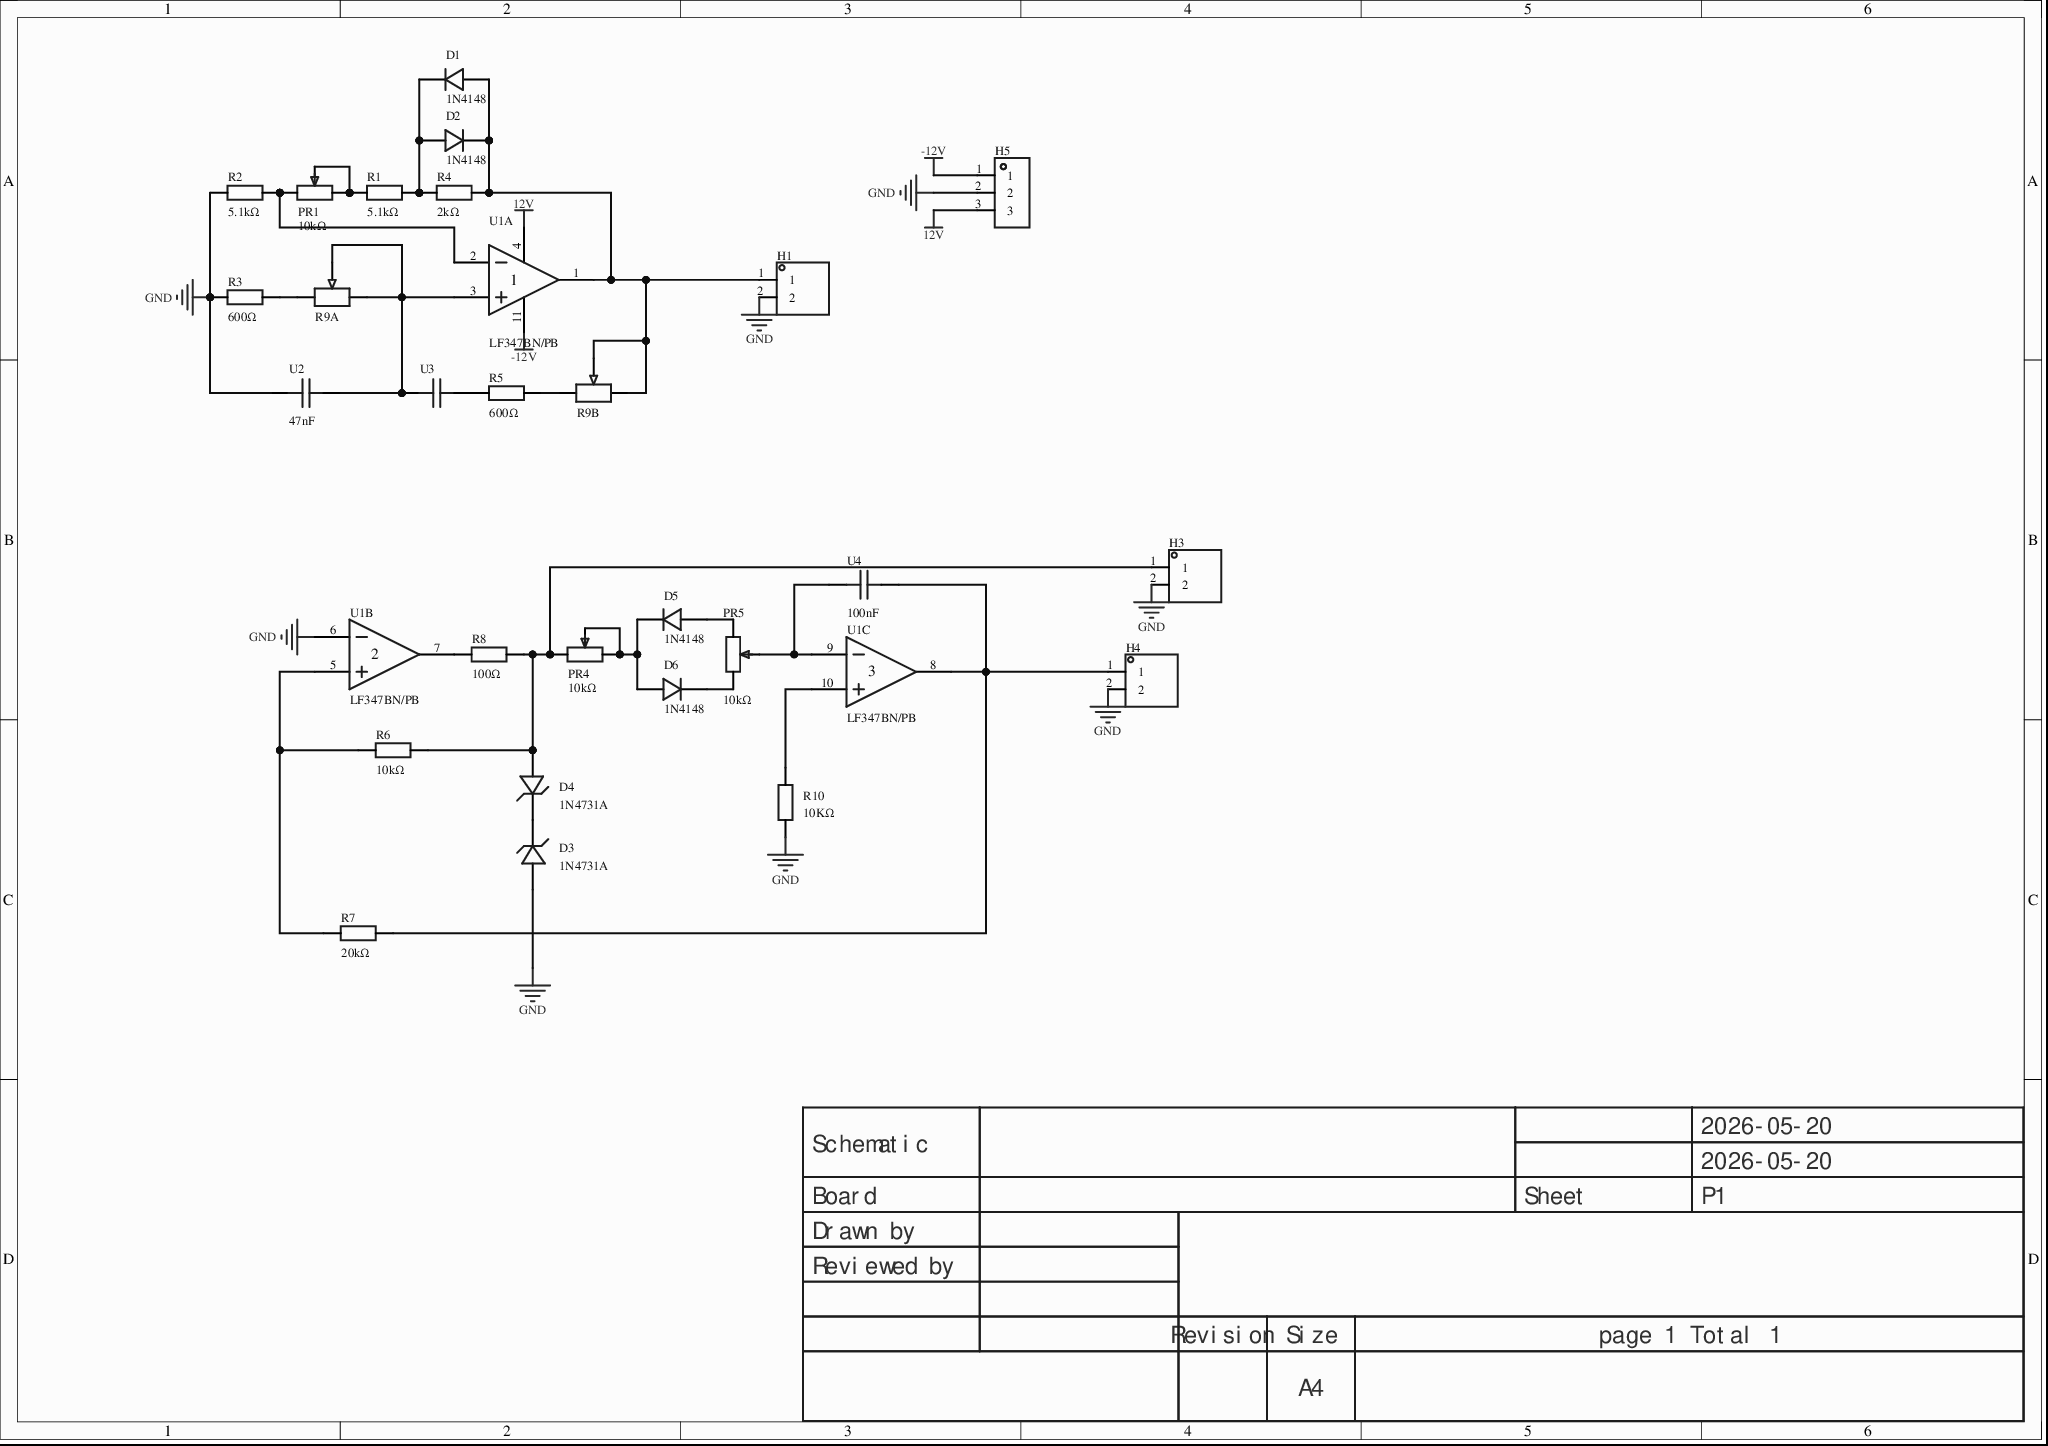
[diagram p0: MISC89085-3.schdoc]
# Altium project MISC89085-2.PrjPcb
1 sheet, 27 parts. Net scope: global (net labels, ports and power ports of the same name join across sheets).
Board file: MISC89085.pcbdoc

## Sheet MISC89085-3.schdoc
size 297 x 209 mm; Version: V1.0; @Project Name: MISC89085; @Update Date: 2026-05-20; @Create Date: 2026-05-20; @Board Name: MISC89085; @Create Time: 18:00:22; @Page Count: 1; @Page No: 1; @Schematic Name: MISC89085; @Update Time: 18:00:22; Size: A4

### Parts
D1  1N4148  [DO-35_BD2.2-L4.0-D0.50_1N4148]
D2  1N4148  [DO-35_BD2.2-L4.0-D0.50_1N4148]
D3  1N4731A  [DO-41_BD2.4-L4.7-P8.70-D0.9-RD]
D4  1N4731A  [DO-41_BD2.4-L4.7-P8.70-D0.9-RD]
D5  1N4148  [DO-35_BD2.2-L4.0-D0.50_1N4148]
D6  1N4148  [DO-35_BD2.2-L4.0-D0.50_1N4148]
H1  (no value)  [HDR-TH_2P-P2.54-V-M-1]
H3  (no value)  [HDR-TH_2P-P2.54-V-M-1]
H4  (no value)  [HDR-TH_2P-P2.54-V-M-1]
H5  (no value)  [HDR-TH_3P-P2.54-V-M]
PR1  10kΩ  [R_3296]
PR4  10kΩ  [R_3296]
PR5  10kΩ  [R_3296]
R1  5.1kΩ  [Res_1/8W]
R2  5.1kΩ  [Res_1/8W]
R3  600Ω  [Res_1/8W]
R4  2kΩ  [Res_1/8W]
R5  600Ω  [Res_1/8W]
R6  10kΩ  [Res_1/8W]
R7  20kΩ  [Res_1/8W]
R8  100Ω  [Res_1/8W]
R9  (no value)  [WH148]  (parts A,B of 2)
R10  10KΩ  [Res_1/8W]
U1  LF347BN/PB  [PDIP-14_L19.6-W6.5-P2.54-LS7.9-BL]  (parts A,B,C of 4)
U2  47nF  [CAP-TH_L5.0-W2.5-P5.00-D1.0]
U3  47nF  [CAP-TH_L5.0-W2.5-P5.00-D1.0]  (value not drawn)
U4  100nF  [CAP-TH_L5.0-W2.5-P5.00-D1.0]

### Nets
12V: H5.3 U1.4(VCC+)
-12V: H5.1 U1.11(VCC-)
GND: D3.2(A) H1.2 H3.2 H4.2 H5.2 R2.1 R3.1 R10.1 U1.6(IN2-) U2.2
NetD1_1: D1.1(A) D2.2(C) H1.1 R4.2 R9.5 R9.6 U1.1(OUT1)
NetD1_2: D1.2(C) D2.1(A) R1.2 R4.1
NetD3_1: D3.1(C) D4.1(C)
NetD4_2: D4.2(A) H3.1 PR4.3 R6.2 R8.2
NetD5_1: D5.1(A) PR5.3
NetD5_2: D5.2(C) D6.1(A) PR4.1 PR4.2
NetD6_2: D6.2(C) PR5.1
NetH4_1: H4.1 R7.2 U1.8(OUT3) U4.1
NetPR1_1: PR1.1 PR1.2 R1.1
NetPR1_3: PR1.3 R2.2 U1.2(IN1-)
NetPR5_2: PR5.2 U1.9(IN3-) U4.2
NetR3_2: R3.2 R9.3
NetR5_1: R5.1 U3.1
NetR5_2: R5.2 R9.4
NetR6_1: R6.1 R7.1 U1.5(IN2+)
NetR8_1: R8.1 U1.7(OUT2)
NetR9_1: R9.1 R9.2 U1.3(IN1+) U2.1 U3.2
NetR10_2: R10.2 U1.10(IN3+)

### Notes on the sheet
- 2026-05-20
- Schematic
- Board
- Sheet
- P1
- Drawn by
- Reviewed by
- Revision
- Size
- A4
- page 1 Total 1

### Library data of the parts
D1 D2 D5 D6 = 1N4148_C9900036548: AddInBom: yes; ModelId: b29439ed7b924f62acded4384188502f0819f05c4eef4c71ace90d822a990e87; ModelTransform: 334.645,87.008,0,0,0,0,0,0,-196.85; Symbol: 1N4148_C9900036548; Device: 1N4148_C9900036548; LCSC Part Name: 1N4148; SupplierPart: C9900036548; ManufacturerPart: 1N4148; Supplier Footprint: LL34; JLCPCB Part Class: Extended Part; Supplier: LCSC; ConvertToPcb: yes; FootprintName: DO-35_BD2.2-L4.0-D0.50_1N4148; ModelName: DO-35_BD2.2-L4.0-D0.50_1N4148
D3 D4 = 1N4731A: Diode configuration: standalone; Zener voltage (nominal): 4.3V; Zener voltage (range): 4.085V~4.515V; Power (Pd): 1W;; Manufacturer: TC(德昌); Symbol: 1N4731A_C261313; AddInBom: yes; ModelId: 6de1e9b71a0d4751b4e9df530304c1a30819f05c4eef4c71ace90d822a990e87; ModelName: DO-41_D2.4-L4.7-P8.70; ModelTransform: 374.016,94.488,0,0,0,0,0,0,-137.795; Reverse Leakage Current (Ir): 10uA@1V; Zener Impedance (Zzt): 9Ω; Device: 1N4731A; LCSC Part Name: 1N4731A; SupplierPart: C261313; ManufacturerPart: 1N4731A; Supplier Footprint: DO-41; JLCPCB Part Class: Extended Part; Datasheet: example.com/20180730/C261314_DA1057BB6837687397320D9A8FF0874A.pdf; Supplier: LCSC; ConvertToPcb: yes; FootprintName: DO-41_BD2.4-L4.7-P8.70-D0.9-RD; Diode Configuration: Standalone; Zener Voltage (Nom): 4.3V; Zener Voltage (Range): 4.085V~4.515V; Power Dissipation: 1W
H1 H3 H4 = HDR-M_2.54_1x2P: Symbol: 210S-1*2P L=11.6MMGold-plated black; ConvertToPcb: yes; ModelId: 79b2e9f2d70a4d68a1b7098f27c6d4c50819f05c4eef4c71ace90d822a990e87; ModelName: HDR-M-2.54_1x2; ModelTransform: 200,100,0,0,0,0,0,0,-118.11; Device: HDR-M_2.54_1x2P; AddInBom: yes; SupplierPart: C124375; Supplier Footprint: 插件; FootprintName: HDR-TH_2P-P2.54-V-M-1
H5 = HDR-M_2.54_1x3P: AddInBom: yes; ModelId: bb473b6d38ff42a99216a4fcdbdcc4cb0819f05c4eef4c71ace90d822a990e87; ModelName: HDR-TH_3P-P2.54-M-LI-1X3P; ModelTransform: 300.03877,100,0,0,0,0,0,0,-118.11; Symbol: HDR-M_2.54_1x3P; Device: HDR-M_2.54_1x3P; ConvertToPcb: yes; FootprintName: HDR-TH_3P-P2.54-V-M; SupplierPart: C2937625; Supplier Footprint: 插件
PR1 PR4 = R_3296: ConvertToPcb: yes; ModelId: b182808559bb43bda9e7de64b64134cb0819f05c4eef4c71ace90d822a990e87; ModelName: 3296W; ModelTransform: 373.98,188.96,590.49,180,0,0,0,0,-140; Symbol: R_3296; Device: R_3296; AddInBom: yes; Supplier Footprint: 直插; FootprintName: R_3296; Value: 10kΩ
PR5 = R_3296: 3D Model: b182808559bb43bda9e7de64b64134cb0819f05c4eef4c71ace90d822a990e87; 3D Model Transform: 373.98,188.96,590.49,180,0,0,0,0,-140; ConvertToPcb: yes; ModelName: 3296W; Symbol: R_3296; Device: R_3296; Supplier Footprint: 直插; Value: 10kΩ; AddInBom: yes; FootprintName: R_3296
R1-R8 R10 = Res_AXIAL-1/8W: Symbol: Resistor; ConvertToPcb: yes; ModelId: b2b5ae7ae4c642178fe0039925c86a3f0819f05c4eef4c71ace90d822a990e87; ModelName: RES-TH_BD1.8-L3.2-P7.20-D0.4; ModelTransform: 282.86,66.88,253.09,0,0,0,0,0,-191; Device: Res_AXIAL-1/8W; AddInBom: yes; Supplier Footprint: 轴向引线; FootprintName: Res_1/8W
  R1 R2: Value: 5.1kΩ
  R3 R5: Value: 600Ω
  R4: Value: 2kΩ
  R6: Value: 10kΩ
  R7: Value: 20kΩ
  R8: Value: 100Ω
  R10: Value: 10KΩ
R9 = WH148: Manufacturer: ALPS Electric; Manufacturer Part: RK0971221Z05; Symbol: WH148_1; Add into BOM: yes; Pin Type: IN; Resistance: 10K; Device: WH148; Convert to PCB: yes; Supplier: LCSC; Supplier Part: C336003; JLCPCB Part Class: Extended library; FootprintName: WH148
U1 = LF347BN/PB: Gain-bandwidth product (GBP): -; Input bias current (Ib): 50pA; Slew rate (SR): 13V/us;; Manufacturer: TI(德州仪器); Relevance: []; AddInBom: yes; ModelId: 9c02f2b186e4457baa67e0f5e04a653b0819f05c4eef4c71ace90d822a990e87; ModelName: PDIP-14_L19.6-W6.5-H5.1-P2.54-LS7.9-BL; ModelTransform: 771.652,311.8104,0,0,0,0,0,0,-118.11; Symbol: LF347BN/PB; Device: LF347BN/PB; LCSC Part Name: LF347BN/PB; SupplierPart: C4370431; ManufacturerPart: LF347BN/PB; Supplier Footprint: PDIP-14; JLCPCB Part Class: Extended Part; Datasheet: example.com/20240130/3238CDA9089C6C1DBA543802052DA4E2.pdf; Supplier: LCSC; ConvertToPcb: yes; FootprintName: PDIP-14_L19.6-W6.5-P2.54-LS7.9-BL; Gain Bandwidth Product(GBP): -; Current - Input Bias(Ib): 50pA; Slew Rate(SR): 13V/us; Operating Temperature: 0℃~+70℃
U2-U4 = 100nF: Symbol: 100NF_C9900015256; AddInBom: yes; ModelId: 08e3d7481fc7486bb1b263873f51e1e10819f05c4eef4c71ace90d822a990e87; ModelName: CAP-TH_BD5.0-W2.5-P5.08; ModelTransform: 224.652,98.425,0,0,0,0,-0.005,0,-137.795; Device: 100nF; LCSC Part Name: 100nF; SupplierPart: C9900015256; Supplier Footprint: CAP-TH_L5.0-W2.5-P5.00-D1.0; JLCPCB Part Class: Extended Part; Supplier: LCSC; ConvertToPcb: yes; FootprintName: CAP-TH_L5.0-W2.5-P5.00-D1.0
  U2 U3: Manufacturer Part: 47nF
  U4: ManufacturerPart: 100nF